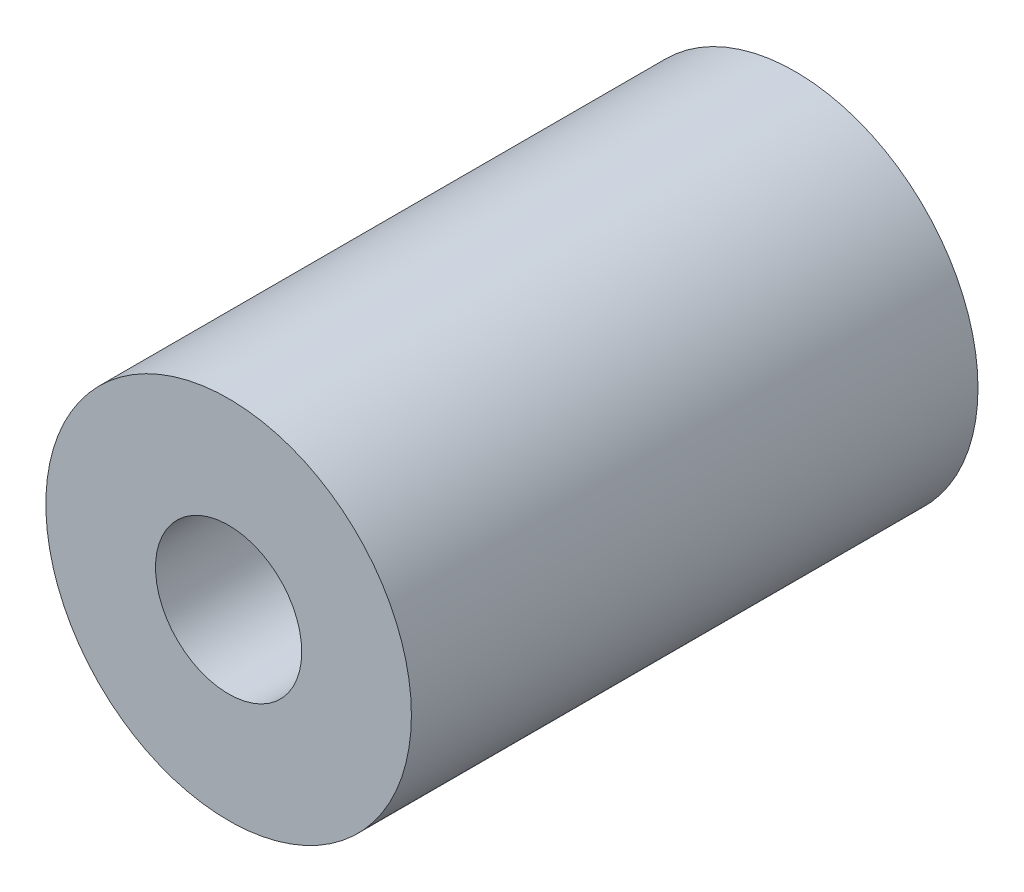
SolidWorks part; units mm, degrees
ref_plane "前视基准面" through (0, 0, 0) normal (0, 0, 1) x (1, 0, 0)
ref_plane "上视基准面" through (0, 0, 0) normal (0, 1, 0) x (1, 0, 0)
ref_plane "右视基准面" through (0, 0, 0) normal (1, 0, 0) x (0, 0, -1)
other "Configuration Table"
sketch "草图1" plane through (0, 0, 0) normal (0, 0, 1) x (1, 0, 0)
  circle A0 centre (0, 0) radius 5
  circle A1 centre (0, 0) radius 2
  dimension "D1" = 10
  dimension "D2" = 4
extrude "凸台-拉伸1" add sketch "草图1" along normal blind 15.5
